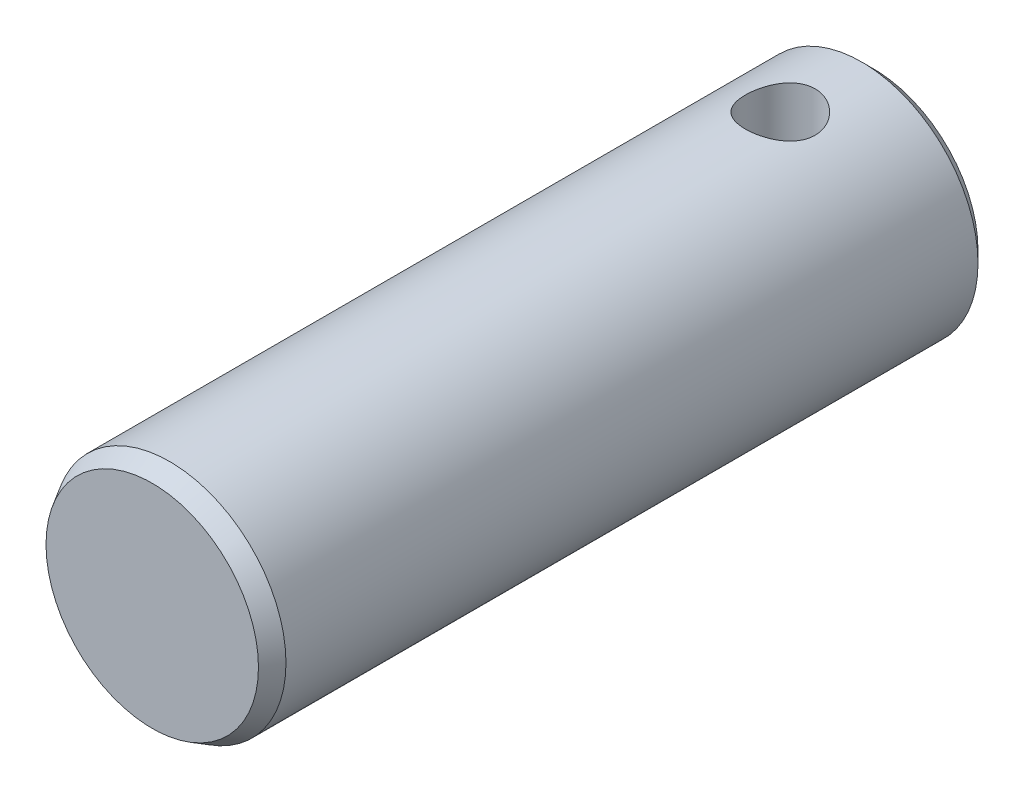
from build123d import *

# Parameters (mm, degrees)
SKETCH_1_R               = 20
EXTRUDE_1_DEPTH          = 124
CHAMFER_1_SIZE           = 3
CHAMFER_1_SIZE2          = 1.732050808
CHAMFER_3_SIZE           = 2
CUT_EXTRUDE_2_DEPTH      = 128.184904765
CUT_EXTRUDE_2_DEPTH_BACK = 128.184904765
SKETCH_3_R               = 6


with BuildPart() as part:
    # 草图1 → 凸台-拉伸1 (new body)
    with BuildSketch(Plane.XY):
        Circle(SKETCH_1_R)
    extrude(amount=EXTRUDE_1_DEPTH)

    # 倒角1
    chamfer_1_edges = [part.edges().sort_by_distance(p)[0] for p in [
        (-20, 0, 124),
    ]]
    chamfer_1_side = [part.faces().sort_by_distance(p)[0] for p in [
        (-20, 0, 62),
    ]]
    chamfer(chamfer_1_edges, length=CHAMFER_1_SIZE, length2=CHAMFER_1_SIZE2, reference=chamfer_1_side[0])

    # 倒角3
    chamfer_3_edges = [part.edges().sort_by_distance(p)[0] for p in [
        (-20, 0, 0),
    ]]
    chamfer(chamfer_3_edges, length=CHAMFER_3_SIZE)

    # 草图3 → 切除-拉伸2 (cut, two sides: drawn at the far end of the back side and taken through both)
    with BuildSketch(Plane(origin=(0, 0, 0), x_dir=(1, 0, 0), z_dir=(0, 1, 0)).offset(-CUT_EXTRUDE_2_DEPTH_BACK)):
        with Locations(Location((0, -16, 0), (0, 0, 270))):
            Circle(SKETCH_3_R)
    extrude(amount=CUT_EXTRUDE_2_DEPTH + CUT_EXTRUDE_2_DEPTH_BACK, mode=Mode.SUBTRACT)


solid = part.part
